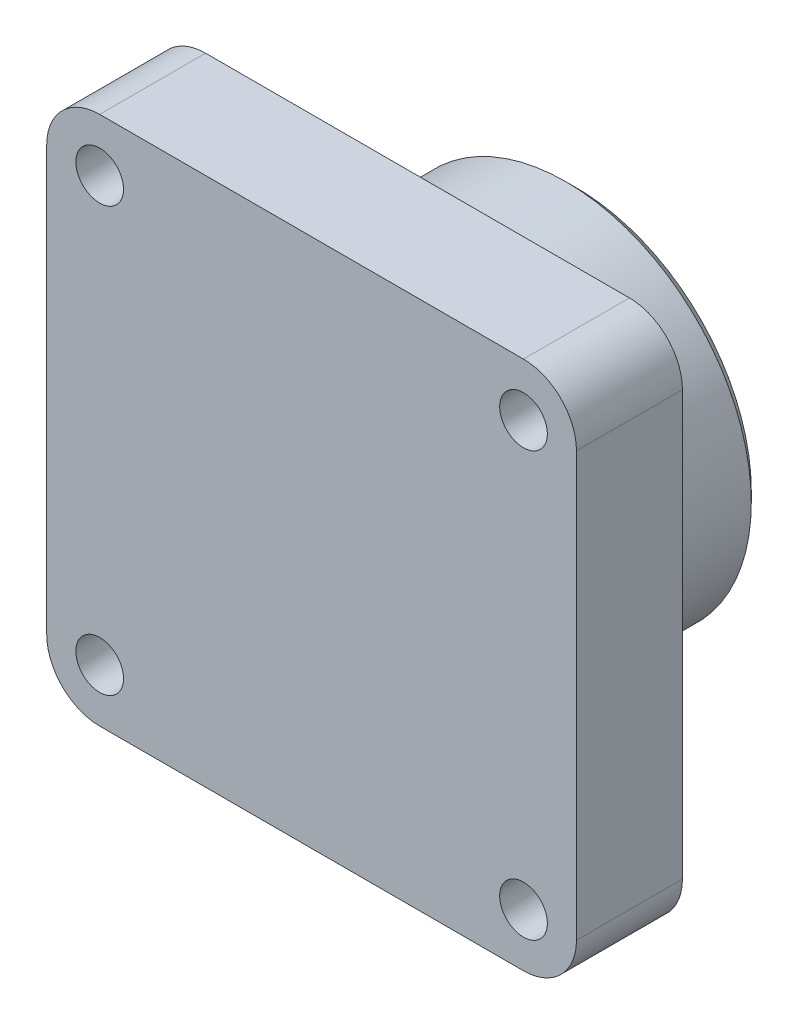
SolidWorks part; units mm, degrees
ref_plane "Front Plane" through (0, 0, 0) normal (0, 0, 1) x (1, 0, 0)
ref_plane "Top Plane" through (0, 0, 0) normal (0, 1, 0) x (1, 0, 0)
ref_plane "Right Plane" through (0, 0, 0) normal (1, 0, 0) x (0, 0, -1)
sketch "Sketch1" plane through (0, 0, 0) normal (0, 0, 1) x (1, 0, 0)
  circle A0 centre (0, 0) radius 12.6
  dimension "D1" = 25.2
extrude "Boss-Extrude1" add sketch "Sketch1" along normal blind 10.8
sketch "Sketch2" plane through (0, 0, 10.8) normal (0, 0, 1) x (1, 0, 0)
  line L1 (-18, -18) -> (18, -18)
  line L2 (-18, -18) -> (-18, 18)
  line L3 (-18, 18) -> (18, 18)
  line L4 (18, -18) -> (18, 18)
  line L5 (-18, -18) -> (18, 18) construction
  line L6 (-18, 18) -> (18, -18) construction
  point P0 (0, 0)
  dimension "D1" = 36
  dimension "D2" = 36
extrude "Boss-Extrude2" add sketch "Sketch2" along normal blind 7.2
fillet "Fillet1" radius 3.6 4 edges at (-18, 18, 14.4) (-18, -18, 14.4) (18, -18, 14.4) (18, 18, 14.4)
chamfer "Chamfer1" distance 0.72 angle 45 1 edges at (12.6, 0, 0)
sketch "Sketch3" plane through (0, 0, 10.8) normal (0, 0, -1) x (-1, 0, 0)
  circle A0 centre (0, 0) radius 12.6
  circle A1 centre (0, 0) radius 14.4
  dimension "D1" = 25.2
  dimension "D2" = 28.8
extrude "Cut-Extrude1" cut sketch "Sketch3" against normal blind 1.08
sketch "Sketch4" plane through (0, 0, 0) normal (0, 1, 0) x (1, 0, 0)
  line L0 (0, 2.7467) -> (0, -20.707) construction
  line L1 (12.6, -11.88) -> (12.6, -0.72) construction
  line L2 (12.06, -6.57) -> (13.14, -6.57)
  line L3 (12.06, -6.57) -> (12.06, -6.03)
  line L4 (12.06, -6.03) -> (13.14, -6.03)
  line L5 (13.14, -6.57) -> (13.14, -6.03)
  line L6 (12.06, -6.57) -> (13.14, -6.03) construction
  line L7 (12.06, -6.03) -> (13.14, -6.57) construction
  point P3 (12.6, -6.3)
  dimension "D1" = 0.54
  dimension "D2" = 0.54
revolve "Cut-Revolve1" cut sketch "Sketch4" angle 360 about L0
sketch "Sketch5" plane through (0, 0, 10.8) normal (0, 0, -1) x (-1, 0, 0)
  line L0 (-14.4, 18) -> (14.4, 18) construction
  line L1 (-14.4, -14.4) -> (14.4, -14.4) construction
  line L2 (-14.4, -14.4) -> (-14.4, 14.4) construction
  line L3 (-14.4, 14.4) -> (14.4, 14.4) construction
  line L4 (14.4, -14.4) -> (14.4, 14.4) construction
  line L5 (-14.4, -14.4) -> (14.4, 14.4) construction
  line L6 (-14.4, 14.4) -> (14.4, -14.4) construction
  line L7 (18, 14.4) -> (18, -14.4) construction
  circle A0 centre (14.4, 14.4) radius 1.62
  circle A1 centre (14.4, -14.4) radius 1.62
  circle A2 centre (-14.4, -14.4) radius 1.62
  circle A3 centre (-14.4, 14.4) radius 1.62
  point P0 (0, 0)
  point P20 (0, 0)
  dimension "D3" = 4
  dimension "D4" = 3.24
  dimension "D5" = 28.8
  dimension "D6" = 28.8
  dimension "D1" = 3.6
  dimension "D2" = 3.6
extrude "Cut-Extrude2" cut sketch "Sketch5" against normal up to surface (7.2 mm away) up to face at (0, 0, 18)
sketch "Sketch6" plane through (0, 0, 0) normal (0, 0, -1) x (-1, 0, 0)
  circle A0 centre (0, 0) radius 8.1
  dimension "D1" = 16.2
extrude "Cut-Extrude3" cut sketch "Sketch6" against normal blind 10.8
